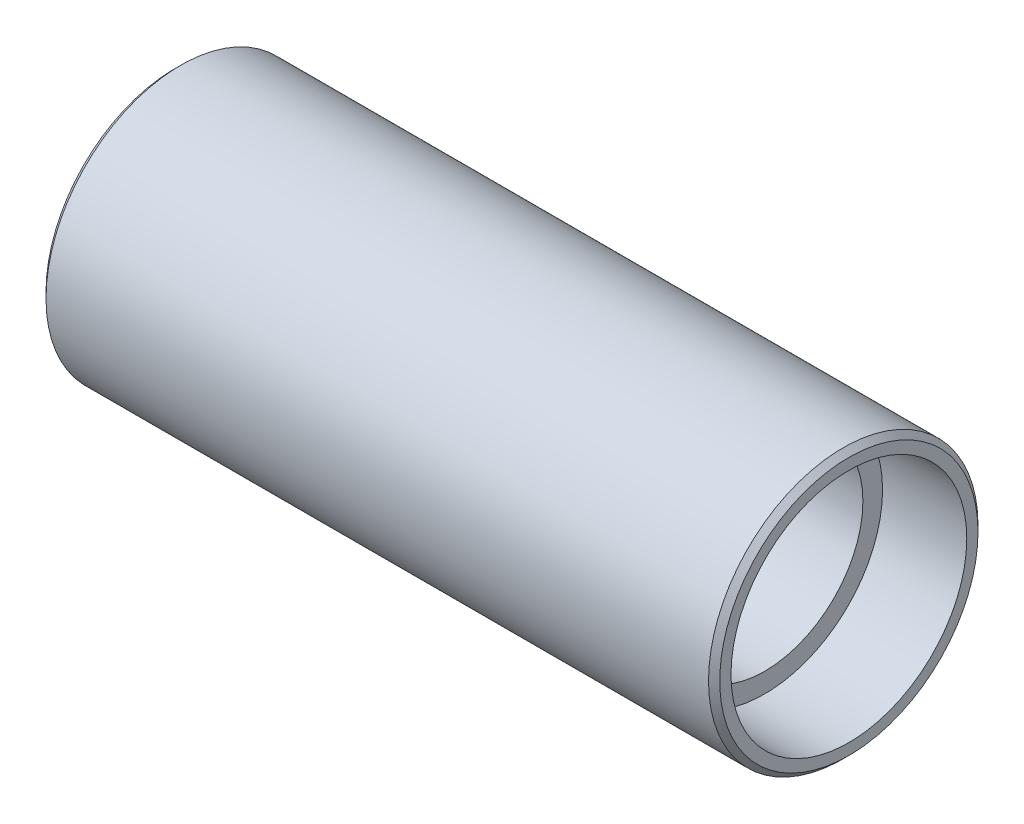
from build123d import *

# Parameters (mm, degrees)
SKETCH1_W          = 120
SKETCH1_H          = 30
SKETCH2_R          = 21
CUT_EXTRUDE1_DEPTH = 15
CUT_EXTRUDE2_START = -15
SKETCH4_R          = 21
CUT_EXTRUDE2_DEPTH = 15
SKETCH5_R          = 17.5
CUT_EXTRUDE3_DEPTH = 114.247516529
SKETCH8_R          = 41.443957881
SKETCH8_R_2        = 24
CUT_EXTRUDE4_DEPTH = 128.279220614
CHAMFER1_SIZE      = 1
CHAMFER3_SIZE      = 1


with BuildPart() as part:
    # Sketch1 → Revolve1 (revolve)
    with BuildSketch(Plane.XY, mode=Mode.PRIVATE) as revolve1_sk:
        with Locations((60, 15)):
            Rectangle(SKETCH1_W, SKETCH1_H)
    revolve(revolve1_sk.sketch.rotate(Axis((0, 0, 0), (-1, 0, 0)), 90), axis=Axis((0, 0, 0), (-1, 0, 0)))

    # Sketch2 → Cut-Extrude1 (cut)
    with BuildSketch(Plane.ZY):
        Circle(SKETCH2_R)
    extrude(amount=-CUT_EXTRUDE1_DEPTH, mode=Mode.SUBTRACT)

    # Sketch4 → Cut-Extrude2 (cut)
    with BuildSketch(Plane(origin=(120, 0, 0), x_dir=(0, 0, -1), z_dir=(1, 0, 0)).offset(CUT_EXTRUDE2_START)):
        with Locations(Location((0, 0, 0), (0, 0, 180))):
            Circle(SKETCH4_R)
    extrude(amount=CUT_EXTRUDE2_DEPTH, mode=Mode.SUBTRACT)

    # Sketch5 → Cut-Extrude3 (cut, through all)
    with BuildSketch(Plane(origin=(105, 0, 0), x_dir=(0, 0, -1), z_dir=(1, 0, 0))):
        Circle(SKETCH5_R)
    extrude(amount=-CUT_EXTRUDE3_DEPTH, mode=Mode.SUBTRACT)

    # Sketch8 → Cut-Extrude4 (cut, through all)
    with BuildSketch(Plane.ZY):
        Circle(SKETCH8_R)
        Circle(SKETCH8_R_2, mode=Mode.SUBTRACT)
    extrude(amount=-CUT_EXTRUDE4_DEPTH, mode=Mode.SUBTRACT)

    # Chamfer1
    chamfer1_edges = [part.edges().sort_by_distance(p)[0] for p in [
        (0, 0, -24),
    ]]
    chamfer(chamfer1_edges, length=CHAMFER1_SIZE)

    # Chamfer3
    chamfer3_edges = [part.edges().sort_by_distance(p)[0] for p in [
        (120, 0, -24),
    ]]
    chamfer(chamfer3_edges, length=CHAMFER3_SIZE)


solid = part.part
